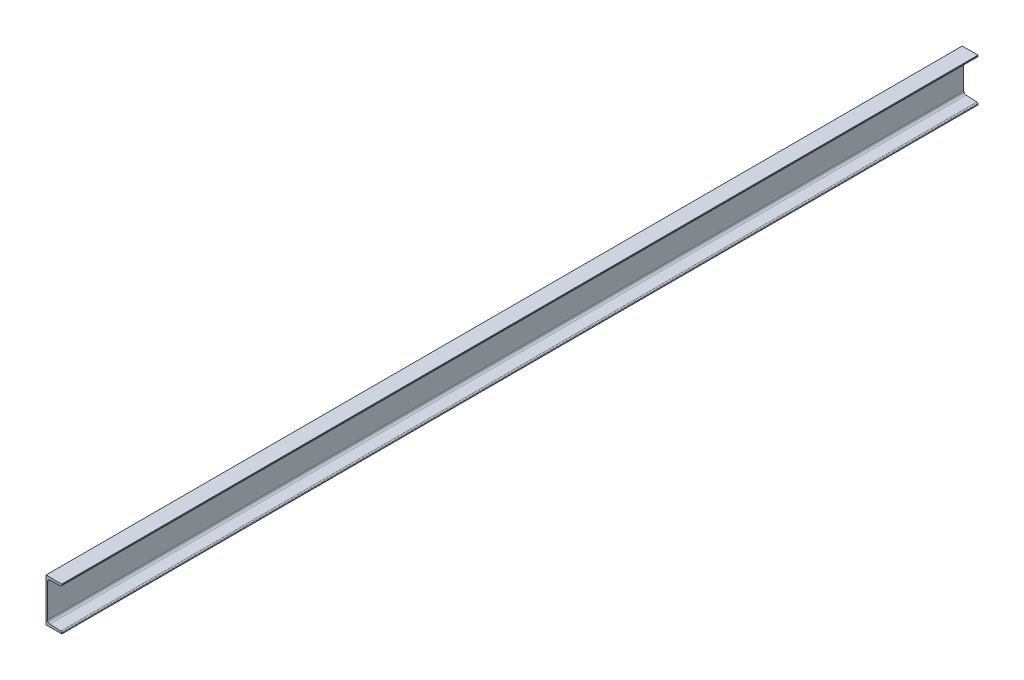
SolidWorks part; units mm, degrees
material "普通碳钢"
ref_plane "Front Plane" through (0, 0, 0) normal (0, 0, 1) x (1, 0, 0)
ref_plane "Top Plane" through (0, 0, 0) normal (0, 1, 0) x (1, 0, 0)
ref_plane "Right Plane" through (0, 0, 0) normal (1, 0, 0) x (0, 0, -1)
sketch "Sketch1" plane through (28.2113, 0, 0) normal (0, 0, 1) x (-1, 0, 0)
  line L0 (28.2113, 0) -> (28.2113, -200)
  line L1 (28.2113, -200) -> (-44.7887, -200)
  line L2 (28.2113, -100) -> (21.2113, -100) construction
  line L3 (21.2113, -177.0757) -> (21.2113, -22.9243)
  line L4 (10.7523, -188.0624) -> (-39.5592, -190.5398)
  line L5 (-44.7887, -196.0332) -> (-44.7887, -200)
  line L6 (21.2113, -187.5473) -> (21.2113, -190.7973) construction
  line L7 (21.2113, -190.7973) -> (-44.7887, -190.7973) construction
  line L8 (-8.2887, -200) -> (-8.2887, -189) construction
  line L9 (-44.7887, -3.9668) -> (-44.7887, 0)
  line L10 (28.2113, 0) -> (-44.7887, 0)
  line L11 (10.7523, -11.9376) -> (-39.5592, -9.4602)
  arc A0 (21.2113, -177.0757) -> (10.7523, -188.0624) centre (10.2113, -177.0757) cw
  arc A1 (10.7523, -11.9376) -> (21.2113, -22.9243) centre (10.2113, -22.9243) cw
  arc A2 (-39.5592, -190.5398) -> (-44.7887, -196.0332) centre (-39.2887, -196.0332) ccw
  arc A3 (-44.7887, -3.9668) -> (-39.5592, -9.4602) centre (-39.2887, -3.9668) ccw
  point P2 (-8.2887, 0)
  point P20 (21.2113, -12.4527)
  point P26 (-44.7887, -9.2027)
  dimension "r" = 11
  dimension "r1" = 5.5
  dimension "h" = 200
  dimension "b" = 73
  dimension "d" = 7
  dimension "t" = 11
  dimension "D5" = 66
  dimension "D6" = 3.25
extrude "Boss-Extrude1" add sketch "Sketch1" along normal mid plane 4241.8
